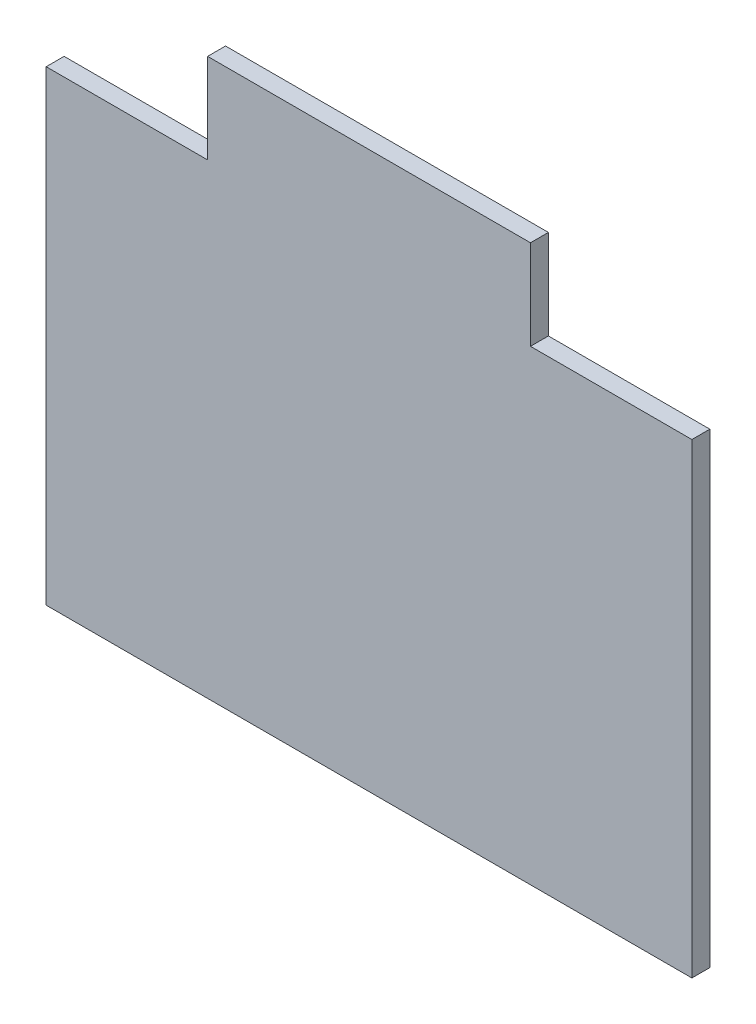
SolidWorks part; units mm, degrees
ref_plane "前视基准面" through (0, 0, 0) normal (0, 0, 1) x (1, 0, 0)
ref_plane "上视基准面" through (0, 0, 0) normal (0, 1, 0) x (1, 0, 0)
ref_plane "右视基准面" through (0, 0, 0) normal (1, 0, 0) x (0, 0, -1)
sketch "草图1" plane through (0, 0, 0) normal (0, 0, 1) x (1, 0, 0)
  line L0 (0, 0) -> (180, 0)
  line L1 (180, 0) -> (180, -130)
  line L2 (0, 0) -> (0, -130)
  line L3 (0, -130) -> (180, -130)
extrude "凸台-拉伸1" add sketch "草图1" along normal blind 5
sketch "草图2" plane through (0, 0, 0) normal (0, 1, 0) x (1, 0, 0)
  line L2 (180, 0) -> (0, 0) construction
  line L4 (45, 0) -> (135, 0)
  line L5 (45, 0) -> (45, -5)
  line L6 (180, -5) -> (0, -5) construction
  line L7 (45, -5) -> (135, -5)
  line L8 (135, -5) -> (135, 0)
extrude "凸台-拉伸2" add sketch "草图2" along normal blind 25
